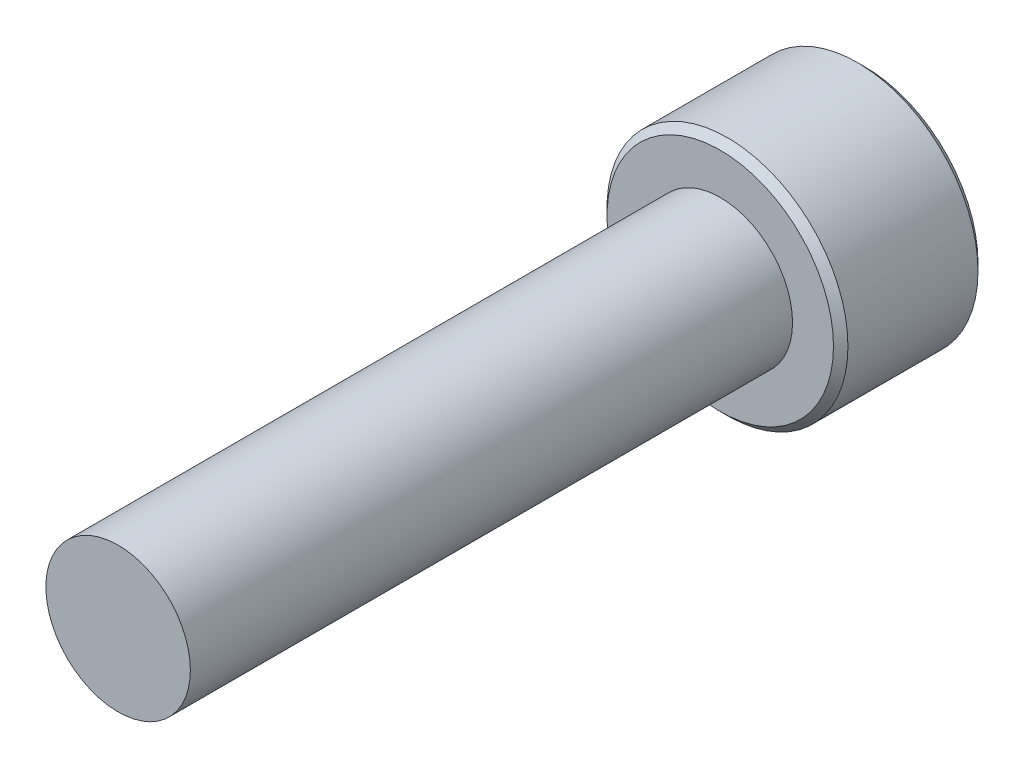
SolidWorks part; units mm, degrees
ref_plane "Front Plane" through (0, 0, 0) normal (0, 0, 1) x (1, 0, 0)
ref_plane "Top Plane" through (0, 0, 0) normal (0, 1, 0) x (1, 0, 0)
ref_plane "Right Plane" through (0, 0, 0) normal (1, 0, 0) x (0, 0, -1)
sketch "Sketch1" plane through (0, 0, 0) normal (0, 0, 1) x (1, 0, 0)
  circle A0 centre (0, 0) radius 5
extrude "Boss-Extrude1" add sketch "Sketch1" along normal blind 6
sketch "Sketch2" plane through (0, 0, 6) normal (0, 0, 1) x (1, 0, 0)
  circle A0 centre (0, 0) radius 3
extrude "Boss-Extrude2" add sketch "Sketch2" along normal blind 25
chamfer "Chamfer1" distance 0.3 angle 45 2 edges at (5, 0, 0) (5, 0, 6)
sketch "Sketch3" plane through (0, 0, 0) normal (0, 0, -1) x (-1, 0, 0)
  line L1 (0, 2.4293) -> (-2.1039, 1.2147)
  line L2 (-2.1039, 1.2147) -> (-2.1039, -1.2147)
  line L3 (-2.1039, -1.2147) -> (0, -2.4293)
  line L4 (0, -2.4293) -> (2.1039, -1.2147)
  line L5 (2.1039, -1.2147) -> (2.1039, 1.2147)
  line L6 (2.1039, 1.2147) -> (0, 2.4293)
  circle A0 centre (0, 0) radius 2.1039 construction
extrude "Cut-Extrude1" cut sketch "Sketch3" against normal blind 3
